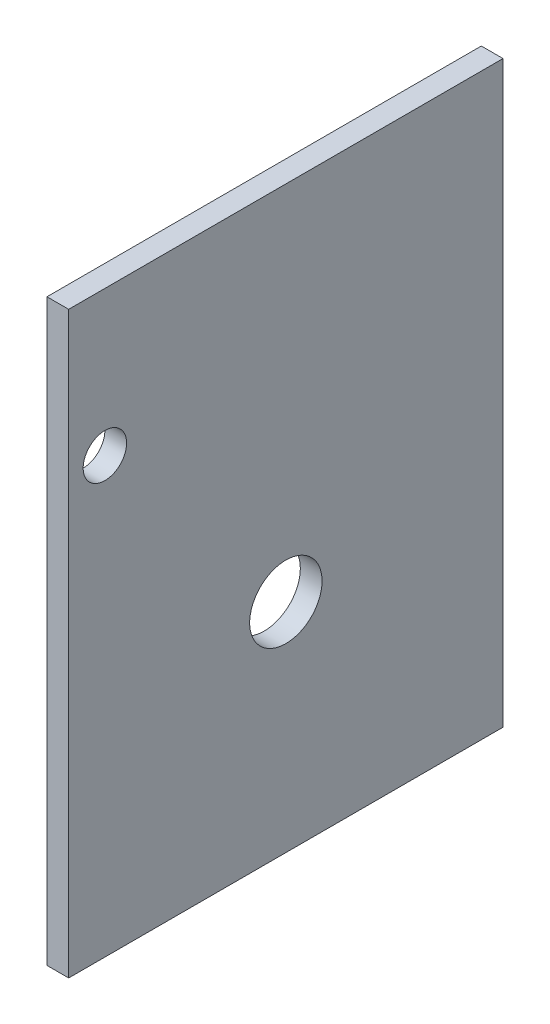
from build123d import *

# Parameters (mm, degrees)
SKETCH1_W           = 60
SKETCH1_H           = 80
SKETCH1_R           = 3
BOSS_EXTRUDE1_DEPTH = 3
SKETCH2_R           = 5
CUT_EXTRUDE1_DEPTH  = 3


with BuildPart() as part:
    # Sketch1 → Boss-Extrude1 (new body)
    with BuildSketch(Plane(origin=(0, 0, 0), x_dir=(0, 0, -1), z_dir=(1, 0, 0))):
        Rectangle(SKETCH1_W, SKETCH1_H)
        with Locations((-25, 20)):
            Circle(SKETCH1_R, mode=Mode.SUBTRACT)
        with Locations((0, -10)):
            Circle(SKETCH1_R, mode=Mode.SUBTRACT)
    extrude(amount=BOSS_EXTRUDE1_DEPTH)

    # Sketch2 → Cut-Extrude1 (cut)
    with BuildSketch(Plane(origin=(3, 0, 0), x_dir=(0, 0, -1), z_dir=(1, 0, 0))):
        with Locations((0, -10)):
            Circle(SKETCH2_R)
    extrude(amount=-CUT_EXTRUDE1_DEPTH, mode=Mode.SUBTRACT)


solid = part.part
